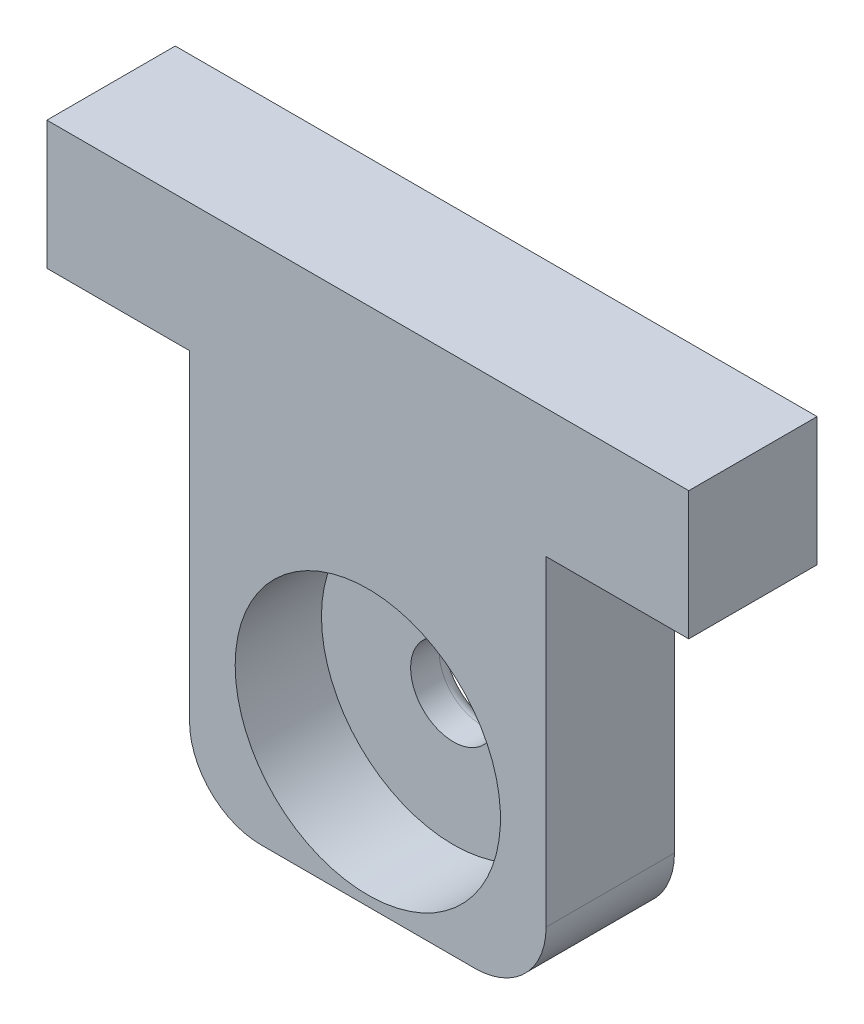
from build123d import *

# Parameters (mm, degrees)
SKETCH_1_W             = 50
SKETCH_1_H             = 120
EXTRUDE_1_DEPTH        = 18
SKETCH_2_W             = 90
SKETCH_2_H             = 18
EXTRUDE_2_DEPTH        = 18
FILLET_1_R             = 10
SKETCH_3_R             = 6
CUT_EXTRUDE_1_DEPTH    = 78.129760793
SKETCH_4_R             = 18.6
SKETCH_4_R_2           = 18.5
CUT_EXTRUDE_2_DEPTH    = 78.129760793
PATTERN_LINEAR_1_COUNT = 2
PATTERN_LINEAR_1_PITCH = 47
FILLET_2_R             = 2
FILLET_3_R             = 2
SKETCH_5_W             = 55.708110293
SKETCH_5_H             = 48.006779115
CUT_EXTRUDE_3_DEPTH    = 78.129760793
FILLET_4_R             = 10
SKETCH_6_R             = 18.6
CUT_EXTRUDE_4_DEPTH    = 12


with BuildPart() as part:
    # 草图1 → 凸台-拉伸1 (new body)
    with BuildSketch(Plane.XY):
        Rectangle(SKETCH_1_W, SKETCH_1_H)
    extrude(amount=EXTRUDE_1_DEPTH)

    # 草图2 → 凸台-拉伸2 (add)
    with BuildSketch(Plane(origin=(0, 60, 0), x_dir=(1, 0, 0), z_dir=(0, 1, 0))):
        with Locations((0, -9)):
            Rectangle(SKETCH_2_W, SKETCH_2_H)
    extrude(amount=-EXTRUDE_2_DEPTH)

    # 圆角1
    fillet_1_edges = [part.edges().sort_by_distance(p)[0] for p in [
        (25, -60, 9),
        (-25, -60, 9),
    ]]
    fillet(fillet_1_edges, radius=FILLET_1_R)

    # 草图3 → 切除-拉伸1 (cut, through all)
    with BuildSketch(Plane(origin=(0, 0, 0), x_dir=(-1, 0, 0), z_dir=(0, 0, -1))):
        with Locations((0, -40)):
            Circle(SKETCH_3_R)
    cut_extrude_1 = extrude(amount=-CUT_EXTRUDE_1_DEPTH, mode=Mode.SUBTRACT)

    # 草图4 → 切除-拉伸2 (cut, through all)
    with BuildSketch(Plane(origin=(0, 0, 0), x_dir=(-1, 0, 0), z_dir=(0, 0, -1))):
        with Locations((0, -40)):
            Circle(SKETCH_4_R)
        with Locations((0, -40)):
            Circle(SKETCH_4_R_2, mode=Mode.SUBTRACT)
    cut_extrude_2 = extrude(amount=-CUT_EXTRUDE_2_DEPTH, mode=Mode.SUBTRACT)


with BuildPart() as cut_extrude_2_piece_1:
    # of the separate pieces the step leaves, piece 1, a body of its own (cut_extrude_2_pieces)
    add(part.part.solids().sort_by_distance((-25, -50, 0))[0])

    # 阵列(线性)1: 切除-拉伸1, 切除-拉伸2 ×2
    with Locations(*[(0, i * PATTERN_LINEAR_1_PITCH, 0) for i in range(1, PATTERN_LINEAR_1_COUNT)]):
        add(cut_extrude_1, mode=Mode.SUBTRACT)
        add(cut_extrude_2, mode=Mode.SUBTRACT)

    # 圆角3
    fillet_3_edges = [cut_extrude_2_piece_1.edges().sort_by_distance(p)[0] for p in [
        (6, 7, 18),
        (6, 7, 0),
        (18.5, 7, 18),
        (18.5, 7, 0),
    ]]
    fillet(fillet_3_edges, radius=FILLET_3_R)


with BuildPart() as cut_extrude_2_piece_2:
    # of the separate pieces the step leaves, piece 2, a body of its own (cut_extrude_2_pieces)
    add(part.part.solids().sort_by_distance((-18.5, -40, 0))[0])

    # 圆角2
    fillet_2_edges = [cut_extrude_2_piece_2.edges().sort_by_distance(p)[0] for p in [
        (6, -40, 18),
        (6, -40, 0),
        (18.5, -40, 18),
        (18.5, -40, 0),
    ]]
    fillet(fillet_2_edges, radius=FILLET_2_R)


with BuildPart() as cut_extrude_3_tool:
    # 草图5 → 切除-拉伸3 (new, through all)
    with BuildSketch(Plane(origin=(0, 0, 0), x_dir=(-1, 0, 0), z_dir=(0, 0, -1))):
        with Locations((-2.854055147, -37.003389558)):
            Rectangle(SKETCH_5_W, SKETCH_5_H)
    extrude(amount=-CUT_EXTRUDE_3_DEPTH)


with BuildPart() as cut_extrude_2_piece_1_1:
    add(cut_extrude_2_piece_1.part)

    # 切除-拉伸3: cut by cut_extrude_3_tool
    add(cut_extrude_3_tool.part, mode=Mode.SUBTRACT)

    # 圆角4
    fillet_4_edges = [cut_extrude_2_piece_1_1.edges().sort_by_distance(p)[0] for p in [
        (25, -13, 9),
        (-25, -13, 9),
    ]]
    fillet(fillet_4_edges, radius=FILLET_4_R)

    # 草图6 → 切除-拉伸4 (cut)
    with BuildSketch(Plane.XY.offset(18)):
        with Locations(Location((0, 7, 0), (0, 0, 180))):
            Circle(SKETCH_6_R)
    extrude(amount=-CUT_EXTRUDE_4_DEPTH, mode=Mode.SUBTRACT)


with BuildPart() as cut_extrude_2_piece_2_1:
    add(cut_extrude_2_piece_2.part)

    # 切除-拉伸3: cut by cut_extrude_3_tool
    add(cut_extrude_3_tool.part, mode=Mode.SUBTRACT)


solid = cut_extrude_2_piece_1_1.part
